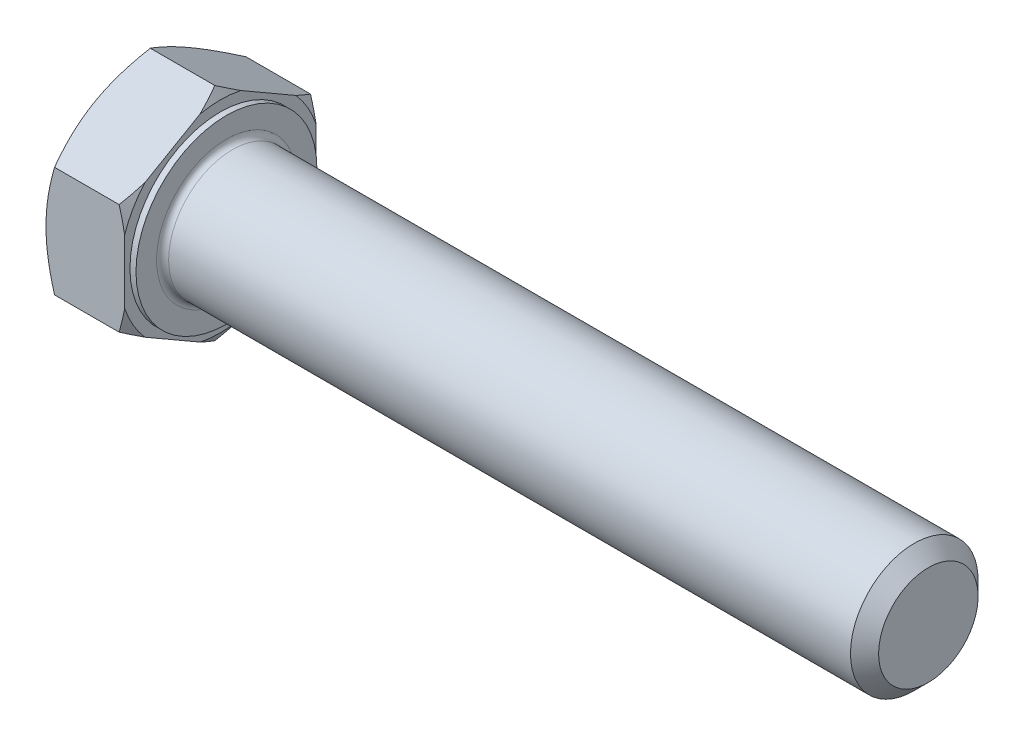
from build123d import *

# Parameters (mm, degrees)
BASE_EXTRUDE_DEPTH = 8.73125
SKETCH4_W          = 0.6
SKETCH4_H          = 11.998522628
CHAMFER_2_SIZE     = 1.4
FILLET_2_R         = 0.6


with BuildPart() as part:
    # Sketch1 → Base-Extrude (new body)
    with BuildSketch(Plane(origin=(0, 0, 0), x_dir=(0, 0, -1), z_dir=(1, 0, 0))):
        Polygon((9.525, 5.499261314), (9.525, -5.499261314), (0, -10.998522628), (-9.525, -5.499261314), (-9.525, 5.499261314), (0, 10.998522628), align=None)
    extrude(amount=BASE_EXTRUDE_DEPTH)

    # Sketch2 → Boss-Revolve1 (revolve)
    with BuildSketch(Plane.XY, mode=Mode.PRIVATE) as boss_revolve1_sk:
        Polygon((0, 0), (78.58125, 0), (78.58125, 5.55625), (78.58125, 6.35), (27.8072, 6.35), (0, 6.35), align=None)
    revolve(boss_revolve1_sk.sketch.rotate(Axis((0, 0, 0), (1, 0, 0)), 90), axis=Axis((0, 0, 0), (1, 0, 0)))

    # Sketch3 → Cut-Revolve1 (revolve, cut)
    with BuildSketch(Plane.XY, mode=Mode.PRIVATE) as cut_revolve1_sk:
        Polygon((0, 9), (4.040598923, 15.998522628), (4.040598923, 20.998522628), (-10, 20.998522628), (-10, 9), align=None)
    revolve(cut_revolve1_sk.sketch.rotate(Axis((0, 0, 0), (1, 0, 0)), 300.000000006), axis=Axis((0, 0, 0), (1, 0, 0)), mode=Mode.SUBTRACT)

    # Sketch5 → Cut-Revolve2 (revolve, cut)
    with BuildSketch(Plane.XY, mode=Mode.PRIVATE) as cut_revolve2_sk:
        Polygon((8.73125, 9), (4.690651077, 15.998522628), (4.690651077, 20.998522628), (14.690651077, 20.998522628), (14.690651077, 9), align=None)
    revolve(cut_revolve2_sk.sketch.rotate(Axis((0, 0, 0), (1, 0, 0)), 90), axis=Axis((0, 0, 0), (1, 0, 0)), mode=Mode.SUBTRACT)

    # Sketch4 → Cut-Revolve3 (revolve, cut)
    with BuildSketch(Plane.XY, mode=Mode.PRIVATE) as cut_revolve3_sk:
        with Locations((8.43125, 14.999261314)):
            Rectangle(SKETCH4_W, SKETCH4_H)
    revolve(cut_revolve3_sk.sketch.rotate(Axis((0, 0, 0), (1, 0, 0)), 90), axis=Axis((0, 0, 0), (1, 0, 0)), mode=Mode.SUBTRACT)

    # Chamfer 2
    chamfer_2_edges = [part.edges().sort_by_distance(p)[0] for p in [
        (78.58125, 0, -6.35),
    ]]
    chamfer(chamfer_2_edges, length=CHAMFER_2_SIZE)

    # Fillet 2
    fillet_2_edges = [part.edges().sort_by_distance(p)[0] for p in [
        (8.73125, 0, -6.35),
    ]]
    fillet(fillet_2_edges, radius=FILLET_2_R)


solid = part.part
